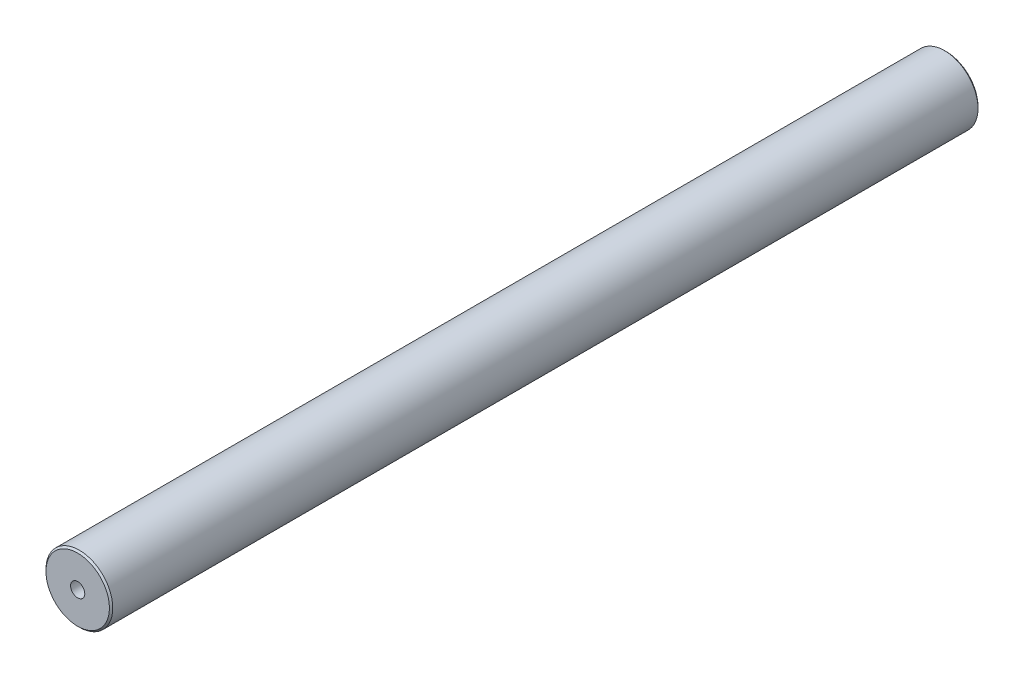
from build123d import *

# Parameters (mm, degrees)
SKETCH_1_R              = 20
EXTRUDE_1_DEPTH         = 520
HOLE_WIZARD_M10_1_D     = 8.5
HOLE_WIZARD_M10_1_DEPTH = 32
HOLE_WIZARD_M10_1_TIP   = 2.553657631
CHAMFER_1_SIZE          = 1
CHAMFER_2_SIZE          = 1
HOLE_WIZARD_M10_2_D     = 8.5
HOLE_WIZARD_M10_2_DEPTH = 24.5
HOLE_WIZARD_M10_2_TIP   = 2.553657631


with BuildPart() as part:
    # 草图1 → 凸台-拉伸1 (new body)
    with BuildSketch(Plane.XY):
        Circle(SKETCH_1_R)
    extrude(amount=EXTRUDE_1_DEPTH)

    # M10 螺纹孔1
    with Locations(Plane(origin=(0, 0, 0), x_dir=(-1, 0, 0), z_dir=(0, 0, -1))):
        with Locations((0, 0)):
            Hole(HOLE_WIZARD_M10_1_D / 2, depth=HOLE_WIZARD_M10_1_DEPTH)
            with Locations((0, 0, -(HOLE_WIZARD_M10_1_DEPTH + HOLE_WIZARD_M10_1_TIP / 2))):  # 118° drill point
                Cone(0, HOLE_WIZARD_M10_1_D / 2, HOLE_WIZARD_M10_1_TIP, mode=Mode.SUBTRACT)

    # 倒角1
    chamfer_1_edges = [part.edges().sort_by_distance(p)[0] for p in [
        (-20, 0, 520),
    ]]
    chamfer(chamfer_1_edges, length=CHAMFER_1_SIZE)

    # 倒角2
    chamfer_2_edges = [part.edges().sort_by_distance(p)[0] for p in [
        (-20, 0, 0),
    ]]
    chamfer(chamfer_2_edges, length=CHAMFER_2_SIZE)

    # M10 螺纹孔2
    with Locations(Plane.XY.offset(520)):
        with Locations((0, 0)):
            Hole(HOLE_WIZARD_M10_2_D / 2, depth=HOLE_WIZARD_M10_2_DEPTH)
            with Locations((0, 0, -(HOLE_WIZARD_M10_2_DEPTH + HOLE_WIZARD_M10_2_TIP / 2))):  # 118° drill point
                Cone(0, HOLE_WIZARD_M10_2_D / 2, HOLE_WIZARD_M10_2_TIP, mode=Mode.SUBTRACT)


solid = part.part
